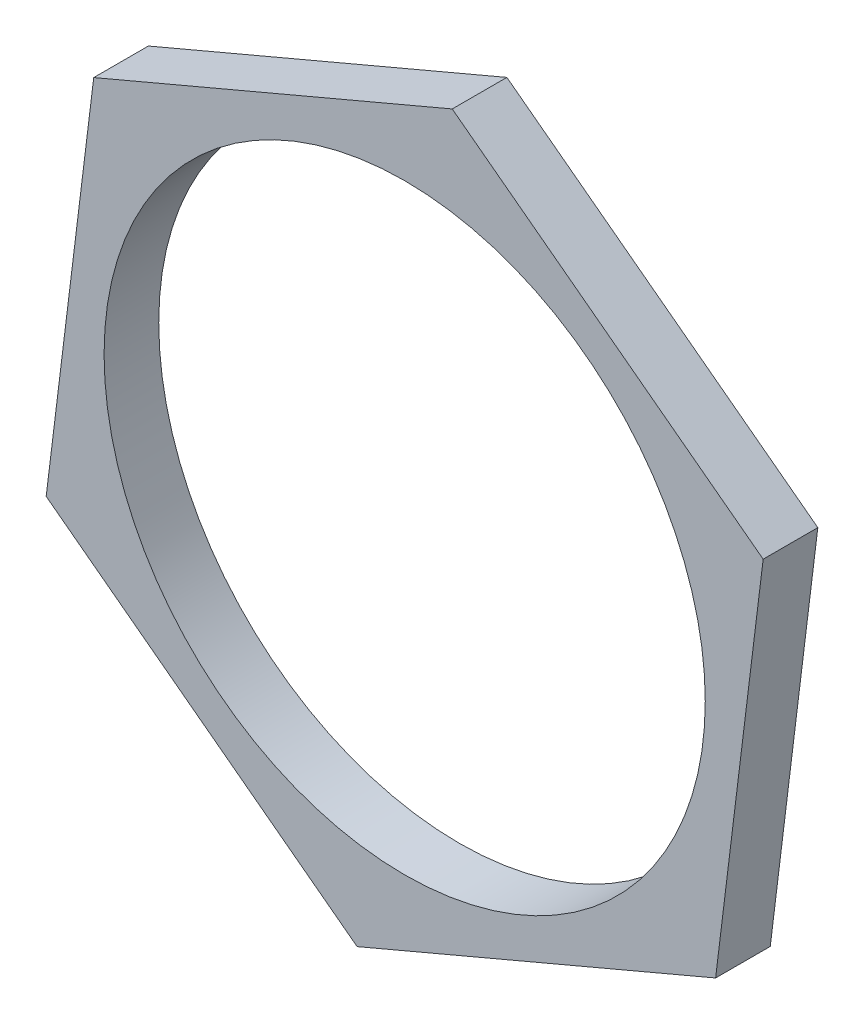
SolidWorks part; units mm, degrees
ref_plane "前视" through (0, 0, 0) normal (0, 0, 1) x (1, 0, 0)
ref_plane "上视" through (0, 0, 0) normal (0, 1, 0) x (1, 0, 0)
ref_plane "右视" through (0, 0, 0) normal (1, 0, 0) x (0, 0, -1)
sketch "草图1" plane through (0, 0, 0) normal (0, 0, 1) x (1, 0, 0)
  line L1 (9.8932, 17.4741) -> (11.6336, 31.6175)
  line L2 (11.6336, 31.6175) -> (0.2553, 40.1963)
  line L3 (0.2553, 40.1963) -> (-12.8634, 34.6319)
  line L4 (-12.8634, 34.6319) -> (-14.6038, 20.4886)
  line L5 (-14.6038, 20.4886) -> (-3.2255, 11.9097)
  line L6 (-3.2255, 11.9097) -> (9.8932, 17.4741)
  circle A0 centre (-1.4851, 26.053) radius 12.3409 construction
  circle A1 centre (-1.4851, 26.053) radius 11
  dimension "D1" = 28.5
extrude "凸台-拉伸1" add sketch "草图1" along normal blind 2
cosmetic thread "装饰螺纹线1" parameters "D2"=24
